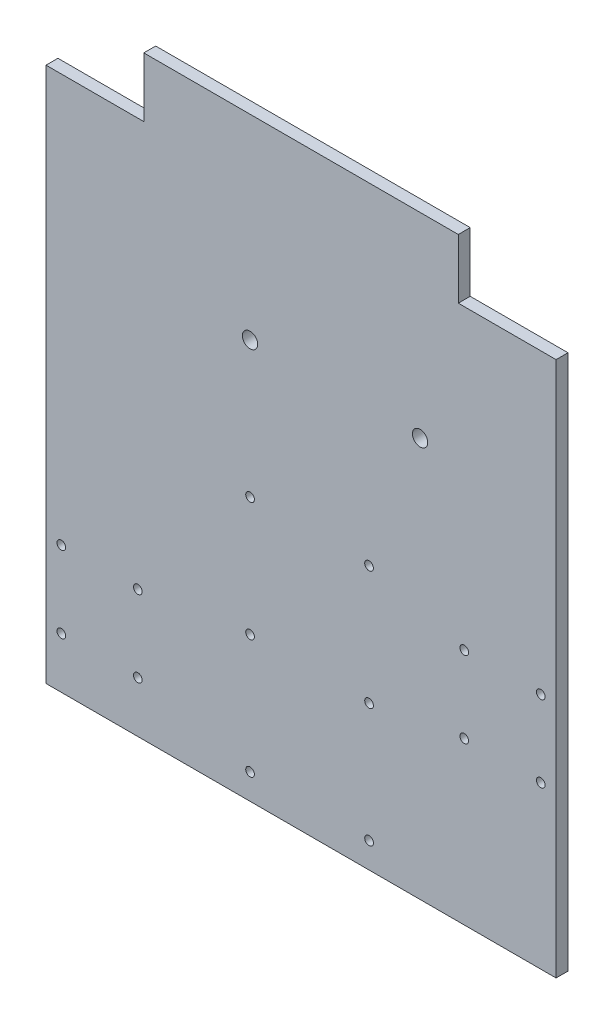
from build123d import *

# Parameters (mm, degrees)
SKETCH_1_R          = 9
EXTRUDE_1_DEPTH     = 14
HOLE_WIZARD_M12_1_D = 10.2


with BuildPart() as part:
    # 草图1 → 凸台-拉伸1 (new body)
    with BuildSketch(Plane.XY):
        Polygon((115, 700), (115, 630), (0, 630), (0, 0), (600, 0), (600, 630), (485, 630), (485, 700), align=None)
        with Locations((440, 470)):
            Circle(SKETCH_1_R, mode=Mode.SUBTRACT)
        with Locations((240, 470)):
            Circle(SKETCH_1_R, mode=Mode.SUBTRACT)
    extrude(amount=EXTRUDE_1_DEPTH)

    # M12 螺纹孔1 (through all)
    with Locations(Plane(origin=(18, 150, 14), x_dir=(1, 0, 0), z_dir=(0, 0, 1))):
        with Locations((0, 0), (90, 0), (0, -90), (90, -90), (474, 130), (564, 130), (474, 40), (564, 40), (222, 160), (362, 160), (222, 20), (362, 20), (222, -120), (362, -120)):
            Hole(HOLE_WIZARD_M12_1_D / 2)


solid = part.part
